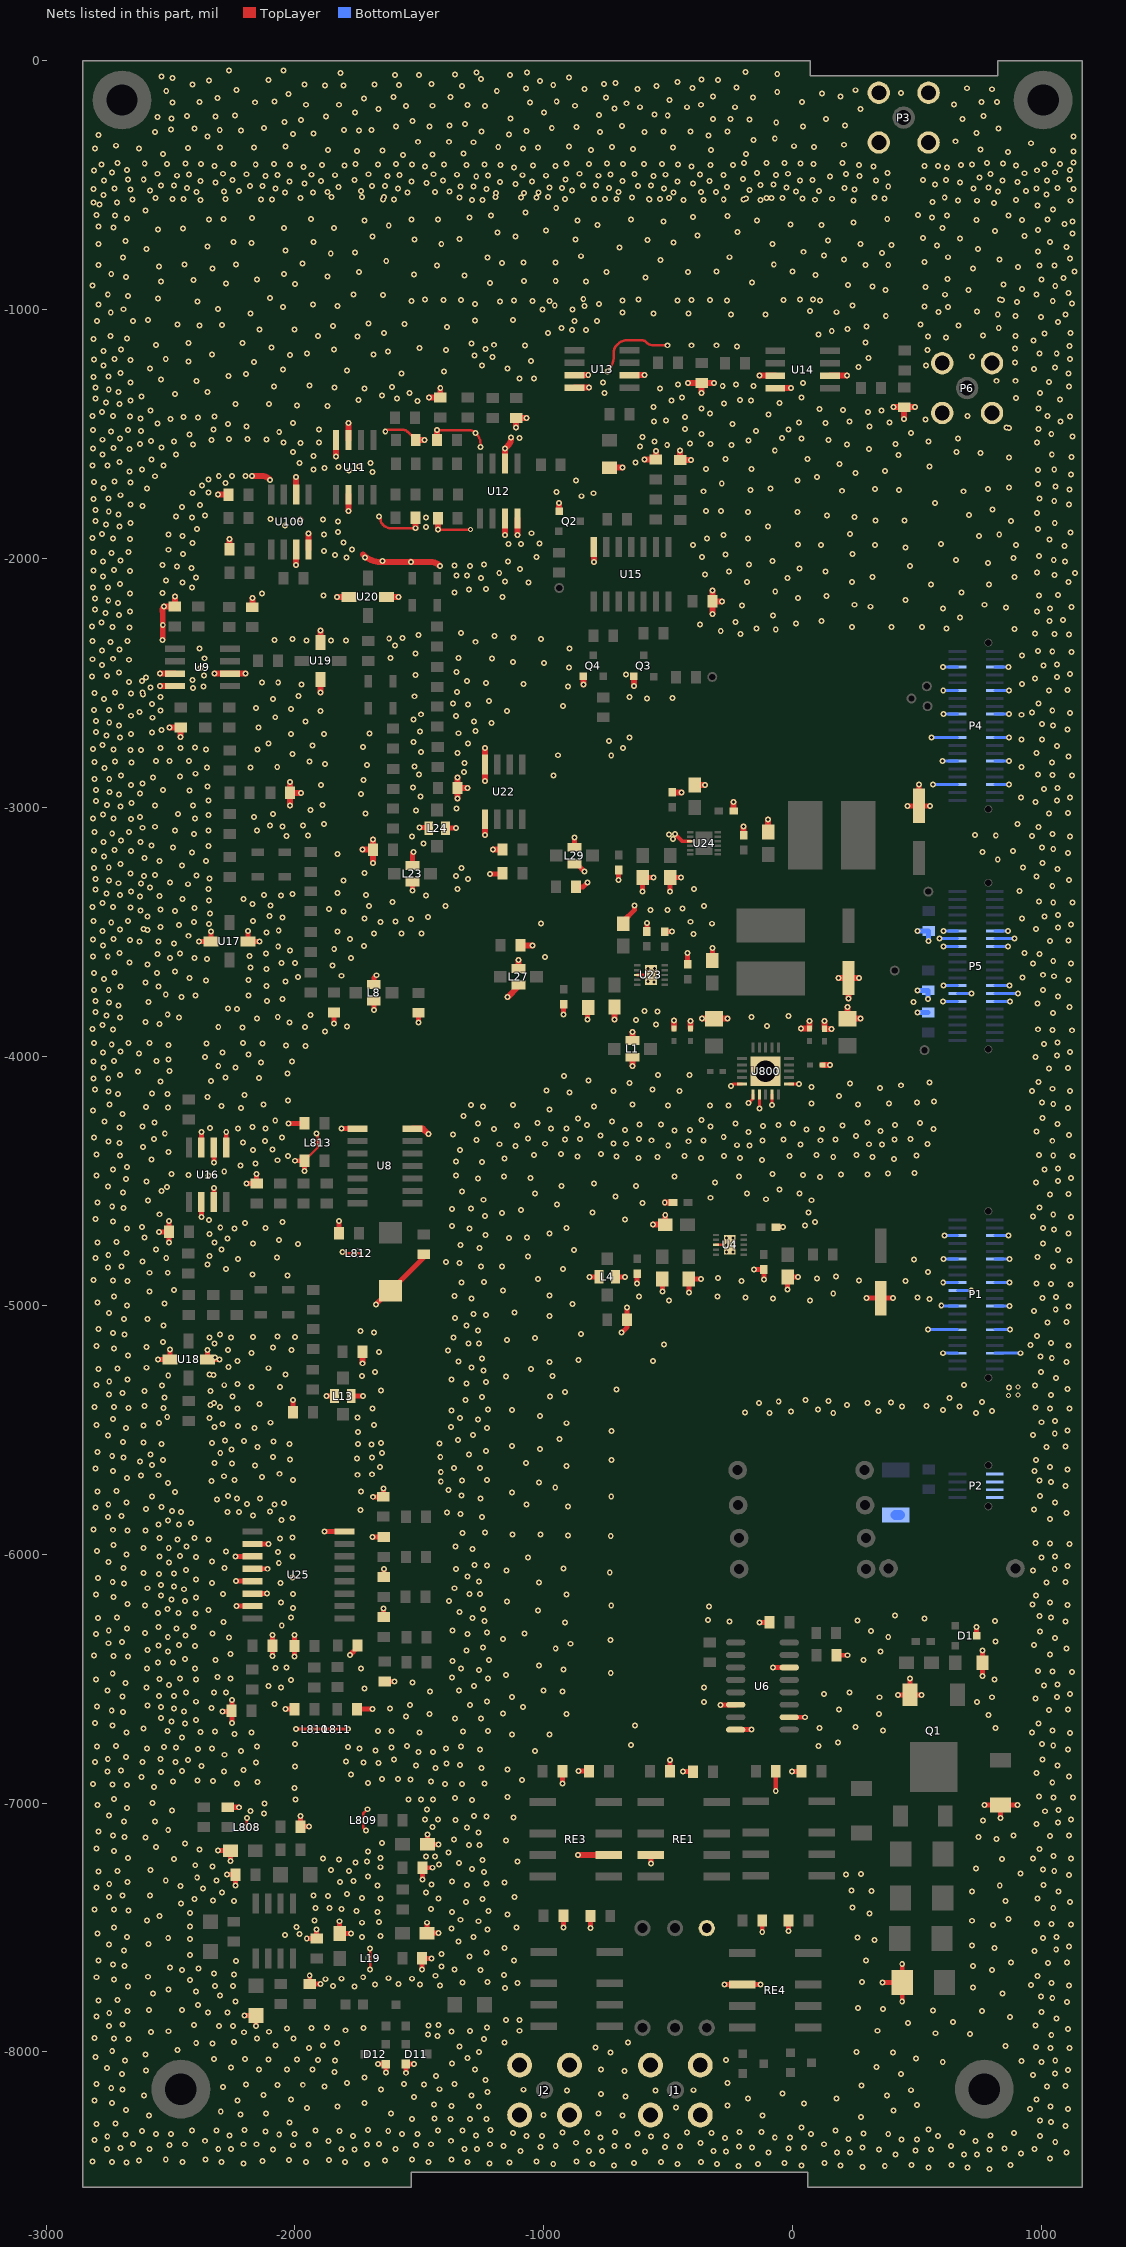
[diagram p0: the nets of this part, all layers, seen from the top]
# Altium PCB MISC109560.PcbDoc (part 3 of 7)
Units mil, origin at the board's own origin, x right, y up, seen from the top; angles counter-clockwise.
Board outline 4015.75 x 8543.31 mil, 4 copper layers (TopLayer, GND, SIG3, BottomLayer); 280 components, 173 nets, 936 pads, 3695 vias.

## Via types
v1: diameter 24, hole 12, TopLayer to BottomLayer, 3659 vias
v2: diameter 20, hole 12, TopLayer to BottomLayer, 32 vias
v3: diameter 40, hole 20, TopLayer to BottomLayer, 4 vias

## Nets (pads, with @x,y where several pads share a name; then routed paths per layer and width w, separated by ;. In a path a pad name is that pad's centre, name@x,y a point inside that pad or via, vN(x,y) a via of type N, cw(c..) or ccw(c..) an arc to the next point about the centre after c; other vN are vias at no path point) (continued)
GND: C5.1 C6.2 C7.1 C8.1 C9.2 C10.2 C11.2 C12.1 C13.2 C14.2 C15.1 C18.2 C20.1 C21.1 C31.1 C32.1 C34.1 C35.1 C36.2 C37.2 C39.2 C40.2 C42.2 C43.1 C44.2 C45.2 C46.2 C47.1 C48.1 C49.2 C50.2 C57.2 C60.2 C61.1 C62.1 C63.1 C64.1 C65.2 C66.1 C70.1 C71.1 C72.2 C73.1 C74.1 C75.1 C80.1 C81.1 C83.2 C84.2 C85.1 C86.2 C88.1 C89.2 C90.2 C93.1 C94.1 C95.2 C96.2 C97.2 C98.2 C99.1 C100.2 C101.2 C102.2 C103.1 C104.2 C105.1 C106.2 C107.2 C109.2 C110.1 C111.1 C112.2 C113.2 C114.1 C115.1 C117.1 C118.2 C119.2 C122.2 C123.2 C124.1 C125.1 C128.1 C129.1 C130.2 C800.2 C801.2 C802.2 C803.2 C804.2 C805.2 C806.2 C809.2 C888.2 D1.3 D2.2 D11.2 D12.1 J1.1 J1.2 J1.3 J1.4 J2.1 J2.2 J2.3 J2.4 L1.2 L1.4 L2.2 L4.2 L4.4 L8.2 L8.4 L13.2 L13.4 L15.2 L16.1 L19.2 L23.2 L23.4 L24.2 L24.4 L27.2 L27.4 L29.2 L29.4 L808.2 L809.2 L810.2 L811.2 L812.2 L813.2 P1.5 P1.6 P1.11 P1.12 P1.17 P1.18 P1.20 P1.23 P1.24 P1.29 P1.30 P1.35 P1.36 P2.1 P2.3 P2.5 P2.7 P3.1 P3.2 P3.3 P3.4 P4.5 P4.6 P4.11 P4.12 P4.17 P4.18 P4.23 P4.24 P4.29 P4.30 P4.35 P4.36 P5.11 P5.12 P5.13 P5.14 P5.15 P5.16 P5.25 P5.26 P5.27 P5.28 P5.29 P5.30 P6.1 P6.2 P6.3 P6.4 Q1.2 Q2.1 Q3.1 Q4.1 R13.2 R14.2 R20.2 R32.2 R53.1 R59.1 R61.1 R71.2 R72.2 R74.1 R80.2 R81.2 R82.1 R83.1 RE1.3 RE3.6 RE4.2 U4.8 U4.11 U6.6 U6.8 U6.10 U6.14 U8.7 U8.8 U9.2 U9.7 U9.8 U11.2 U11.7 U11.8 U12.2 U12.7 U12.8 U13.2 U13.7 U13.8 U14.2 U14.7 U14.8 U15.14 U16.2 U16.3 U16.5 U16.6 U16.7 U17.2 U17.4 U18.2 U18.4 U19.2 U19.4 U20.2 U20.4 U22.4 U22.5 U23.8 U23.11 U24.9 U25.2 U25.3 U25.4 U25.5 U25.6 U25.7 U25.16 U100.2 U100.7 U100.8 U800.5 U800.6 U800.7 U800.9 U800.11 U800.21 | length 17582.9
  TopLayer w10: L808.2@-2193.26,-7104.89 v1(-2193.26,-7059.26) ; C89.2@-1961.96,-4419.31 -1908.26,-4365.61 L813.2@-1908.26,-4352.89 ; v1(-1914,-4310.31) -1908.26,-4316.05 L813.2@-1908.26,-4352.89 ; L813.2@-1908.26,-4339.11 L813.2@-1908.26,-4352.89 ; v1@-1803.43,-4790.57 L812.2@-1749.85,-4790.57 L812.2@-1736.07,-4790.57 ; v1(-1714,-7110) -1725.74,-7098.26 L809.2@-1725.74,-7063.11 -1725.74,-7042.74 v1(-1708,-7025) ; v1(-1698.26,-7669.74) L19.2@-1698.26,-7617.11 v1(-1698.26,-7584.74) ; v1@-1656,-1840.17 ccw(c-1621.86,-1840.17) -1646,-1864.31 ccw(c-1613.19,-1831.5) -1613.19,-1877.9 v1(-1516.41,-1877.9) ; v1@-1638,-1488.31 cw(c-1623.51,-1502.79) -1623.51,-1482.31 -1566,-1482.31 cw(c-1566,-1507.78) -1547.99,-1489.77 C62.1@-1514.41,-1523.35 ccw(c-1539.64,-1523.35) C62.1@-1521.8,-1505.51 ; v1(-1428.41,-1483.9) -1298.13,-1483.9 cw(c-1298.13,-1519.44) -1273,-1494.31 cw(c-1318.87,-1540.18) -1254,-1540.18 v1@-1254,-1552.31 ; v1@-1423.59,-1882.31 ccw(c-1423.59,-1885.72) v1(-1426,-1883.31) v2(-1294,-1883.31) ; v1@-743,-1244.68 ccw(c-800.94,-1186.74) -719,-1186.74 -719,-1171.68 cw(c-677.96,-1171.68) -706.98,-1142.66 -702,-1137.68 cw(c-665.79,-1173.89) -665.79,-1122.68 -605.9,-1122.68 cw(c-605.9,-1146.58) -589,-1129.68 ccw(c-557.62,-1098.29) -557.62,-1142.68 v1(-503,-1142.68) ; U4.8@-308.14,-4756.94 U4.11@-252.57,-4756.94
  TopLayer w12: v1(-1994.74,-6703.26) -1811,-6703.26 ; L811.2@-1822.11,-6703.26 -1811,-6703.26 ; v1(-1786.74,-6703.26) -1811,-6703.26 ; U23.8@-625.14,-3672.94 U23.11@-590.06,-3672.94 ; -444,-3134 -442.55,-3135.45 -441.55,-3135.45 ; v1(-248,-4119) -239.67,-4110.67 U800.5@-203,-4110.67 ; v1(-177,-4188) -159.69,-4170.69 U800.6@-159.69,-4153.98 ; v1(-134.1,-4209.9) U800.7@-134.1,-4153.98 ; v1(-82.92,-4194.92) U800.9@-82.92,-4153.98 ; U800.11@-14.02,-4110.67 v1(26.33,-4110.67)
  TopLayer w13: -441.55,-3135.45 U24.9@-411.41,-3135.45
  TopLayer w16: v1(-472,-3106) -444,-3134
  TopLayer w20: v1(-2549.55,-5217.72) U18.4@-2501.92,-5217.72 v1(-2501.92,-5178.35) ; v1(-2545.96,-4705.31) R53.1@-2505.96,-4705.31 ; v1(-2505.96,-4748.31) R53.1@-2505.96,-4705.31 ; v1(-2505.96,-4662.31) R53.1@-2505.96,-4705.31 ; v1(-2385.59,-3537.72) U17.4@-2337.96,-3537.72 v1(-2337.96,-3498.27) ; v1(-2375.92,-4646.27) U16.2@-2375.92,-4585.72 ; U16.7@-2375.92,-4365.72 v1(-2375.92,-4304.35) ; v1(-2351.92,-5180.27) U18.2@-2351.92,-5217.72 v1(-2303.37,-5217.72) ; U16.3@-2325.92,-4585.72 v1(-2325.92,-4528.27) ; v1(-2325.92,-4427.27) U16.6@-2325.92,-4365.72 ; v1(-2308.89,-7191.41) C86.2@-2259.26,-7191.41 v1(-2259.26,-7233.22) ; v1(-2290.76,-6632.31) R82.1@-2253.29,-6632.31 ; U16.5@-2275.92,-4365.72 v1(-2275.92,-4303.27) ; v1(-2273.48,-7288) C83.2@-2238.48,-7288 v1(-2238.48,-7332) ; v1(-2253.29,-6679.21) R82.1@-2253.29,-6632.31 ; v1(-2253.29,-6585.77) R82.1@-2253.29,-6632.31 ; v1(-2238.61,-6008.69) U25.3@-2170.71,-6008.69 ; v1(-2236.24,-6108.69) U25.5@-2170.71,-6108.69 ; v1(-2234.24,-6208.69) U25.7@-2170.71,-6208.69 ; v1(-2201.89,-7853.41) R61.1@-2156.44,-7853.41 v1(-2156.44,-7894.96) ; v1(-2193.96,-4510.31) C47.1@-2153.96,-4510.31 v1(-2153.96,-4472.31) ; v1(-2187.96,-3495.35) U17.2@-2187.96,-3537.72 v1(-2141.41,-3537.72) ; U25.6@-2170.71,-6158.69 v1(-2111.24,-6158.69) ; U25.4@-2170.71,-6058.69 v1(-2109.24,-6058.69) ; U25.2@-2170.71,-5958.69 v1(-2106.24,-5958.69) ; v1(-2090.71,-6409.79) -2090.71,-6396.01 ; R83.1@-2090.71,-6367.69 -2090.71,-6396.01 ; v1(-2090.71,-6324.23) -2090.71,-6396.01 ; v1(-2037.93,-6623.01) C105.1@-2000.93,-6623.01 ; v1(-2025,-4270) -1995.65,-4270 -1994.96,-4269.31 C50.2@-1960.96,-4269.31 ; C64.1@-2007,-5429.96 v1(-2007,-5380.96) ; v1(-2001.93,-6412.01) C128.1@-2001.93,-6369.01 v1(-2001.93,-6324.01) ; v1(-1999.96,-4419.31) C89.2@-1961.96,-4419.31 v1(-1961.96,-4461.31) ; v1(-1978.48,-7052) R74.1@-1978.48,-7095 v1(-1943.48,-7095) ; v1(-1952.48,-7544) C75.1@-1912.48,-7544 v1(-1912.48,-7508) ; v1(-1940.44,-7692.96) R59.1@-1940.44,-7727.41 v1(-1896.89,-7727.41) ; v1(-1881,-5908.69) U25.16@-1800.71,-5908.69 ; v1(-1873.83,-5364.83) L13.2@-1840.46,-5364.83 ; v1(-1842.59,-3868.72) C48.1@-1842.59,-3826.27 ; C104.2@-1822.96,-4711.31 v1(-1822.96,-4661.04) ; v1(-1820.48,-7475) C71.1@-1820.48,-7524 v1(-1775.48,-7524) ; v1(-1812,-4290.35) U8.8@-1748.37,-4290.35 ; v1(-1778.93,-6405.01) C129.1@-1747.93,-6374.01 ; L13.4@-1773.54,-5364.83 v1(-1725.83,-5364.83) ; C90.2@-1749.93,-6623.01 v1(-1688.93,-6623.01) ; v1(-1687.52,-5931.42) C102.2@-1643.89,-5931.42 ; v1(-1685.34,-5769.42) C96.2@-1644.89,-5769.42 v1(-1644.89,-5736.05) ; v1(-1682.83,-3812.83) L8.4@-1682.83,-3777.46 ; L8.2@-1682.83,-3710.54 -1682.83,-3684.83 v1(-1672,-3674) ; v1(-1675,-4997) -1619.16,-4941.16 C49.2@-1616,-4941.16 -1483,-4808.16 C888.2@-1483,-4795 ; v1(-1665.48,-8049) D12.1@-1634.48,-8049 v1(-1634.48,-8083) ; C118.2@-1643.93,-6252.01 v1(-1643.93,-6218.01) ; C109.2@-1642.89,-6092.42 v1(-1642.89,-6060.05) ; C130.2@-1639.93,-6511.01 v1(-1599.93,-6511.01) ; v1(-1554.26,-8083.78) D11.2@-1554.26,-8048.69 v1(-1521.79,-8048.69) ; v1(-1527.83,-3333.83) L23.4@-1527.83,-3299.46 ; L23.2@-1527.83,-3232.54 v1@-1527.83,-3182.14 ; v1(-1503.43,-3864.61) C123.2@-1503.43,-3824.61 ; v1(-1500,-3081) L24.4@-1464.24,-3081 ; v1(-1488.48,-7668) C74.1@-1488.48,-7624 v1(-1450.48,-7624) ; v1(-1487.48,-7307) C72.2@-1487.48,-7260 v1(-1447.48,-7260) ; v1(-1468.48,-7481) C70.1@-1468.48,-7523 v1(-1422.48,-7523) ; v1(-1467.48,-7126) C73.1@-1467.48,-7166 v1(-1423.48,-7166) ; L24.2@-1395.54,-3082.78 v1@-1353.78,-3082.78 ; v1(-1216,-3268) C125.1@-1169.31,-3268 ; v1(-925,-6920.59) C32.1@-925,-6872.59 ; v1(-921,-7500.59) C39.2@-921,-7453.59 ; v1(-920,-3832) C98.2@-920,-3790 ; L29.4@-876.83,-3226.46 -867.54,-3226.46 v1(-837,-3257) ; L29.2@-876.83,-3159.54 v1(-876.83,-3119.83) ; C115.1@-871,-3319 -842,-3319 v1(-825,-3302) ; v1(-861.41,-6872) C31.1@-817.66,-6872 ; v1(-824,-3851) -824,-3805.31 C93.1@-822,-3803.31 ; v1(-816.17,-4885.83) L4.2@-778.46,-4885.83 ; v1(-812.96,-7501.55) C40.2@-812.96,-7454 ; L4.4@-711.54,-4885.83 v1(-672.83,-4885.83) ; v1(-699,-3291) C113.2@-699,-3251 ; v1(-687,-5110) -665,-5088 C13.2@-665,-5059 v1(-665,-5009) ; C101.2@-680,-3467 -680,-3456 -635,-3411 v1(-635,-3393) ; v1(-625,-4912) C11.2@-625,-4873 ; v1(-603,-3337) C114.1@-603,-3282 v1(-559,-3282) ; R72.2@-586,-3498 v1(-586,-3464) ; v1(-569.66,-7242.25) RE1.3@-569.66,-7208.6 ; v1(-524,-4944) C12.1@-524,-4895 ; R71.2@-514,-3499 v1(-484,-3499) ; C21.1@-493,-6871.59 v1(-493,-6826.59) ; v1(-492,-3337) C110.1@-492,-3282 v1(-449,-3282) ; v1(-440,-6873.59) C20.1@-401,-6873.59 ; C95.2@-422,-3630 v1(-422,-3584) ; v1(-417,-4948) C7.1@-417,-4895 v1(-369,-4895) ; C94.1@-323,-3615 v1(-323,-3565) ; v1(-289.69,-6605.31) U6.6@-229,-6605.31 ; v1(-273.98,-7728.57) RE4.2@-202,-7728.57 v1(-129.02,-7728.57) ; U6.8@-229,-6705.31 v1(-165.31,-6705.31) ; v1(-156,-4856) C9.2@-116,-4856 v1(-116,-4897) ; v1(-134,-6273.69) C15.1@-93,-6273.69 ; v1(-122.26,-7517.33) C35.1@-122.26,-7472 ; v1(-79.69,-6455.31) U6.14@-13.6,-6455.31 ; v1(-68,-6952.59) C37.2@-68,-6872.59 ; R13.2@-67,-4686 v1(-39,-4686) ; v1(-20,-4936) C8.1@-20,-4887 v1(22,-4887) ; v1(-17.26,-7514.33) C34.1@-17.26,-7472 ; U6.10@-13.6,-6655.31 v1(48.69,-6655.31) ; v1(-2,-6872.59) C36.2@35,-6872.59 ; C18.2@175.81,-6406.2 v1(220.51,-6406.2) ; v1(296.76,-4971.24) C10.2@354,-4971.24 v1(403.24,-4971.24) ; v1(360.31,-7720.99) D2.2@440.22,-7720.99 ; v1(423,-6565) Q1.2@472,-6565 ; v1(440.22,-7796.53) D2.2@440.22,-7720.99 ; v1(440.22,-7647.53) D2.2@440.22,-7720.99 ; v1(462,-2993) C117.1@508,-2993 ; v1(472,-6499) Q1.2@472,-6565 ; v1(508,-2908) C117.1@508,-2993 ; v1(517,-6565) Q1.2@472,-6565 ; v1(552,-2993) C117.1@508,-2993 ; D1.3@739,-6328 v1(739,-6293) ; L2.2@762.78,-6436.31 v1(762.78,-6386.22) ; v1(763,-6488.91) L2.2@763,-6444 ; v1(771,-7008) C6.2@835,-7008 ; v1(835,-7061) C6.2@835,-7008 ; v1(903,-7008) C6.2@835,-7008
  TopLayer w24: v1(-2543.04,-2462.27) U9.7@-2481.59,-2462.27 ; v1(-2541.96,-2512.27) U9.8@-2481.59,-2512.27 ; v1@-2531,-2323.31 -2531,-2214.09 ccw(c-2537.83,-2214.09) -2533,-2209.26 ; v1(-2503.59,-2677.72) C66.1@-2458.96,-2677.72 v1(-2458.96,-2717.27) ; v1(-2482.59,-2151.72) C42.2@-2482.59,-2192.27 v1(-2525.96,-2192.27) ; v1(-2322.96,-2462.27) U9.2@-2261.59,-2462.27 v1(-2197.96,-2462.27) ; v1(-2309.59,-1742.72) C43.1@-2265.96,-1742.72 ; C809.2@-2269,-7017 v1(-2224,-7017) ; C61.1@-2263,-1962.31 v1(-2263,-1921.31) ; v1(-2172,-1667.31) -2133.38,-1667.31 cw(c-2133.38,-1711.69) v1@-2102,-1680.31 ; C60.2@-2170.59,-2195.27 v1(-2170.59,-2158.72) ; v1(-2019,-2992.31) C65.2@-2019,-2941.31 ; v1(-2019,-2898.31) C65.2@-2019,-2941.31 ; v1(-1994.96,-2025.27) U100.7@-1994.96,-1962.72 ; U100.2@-1994.96,-1742.72 v1(-1994.96,-1672.35) ; v1(-1975,-2941.31) C65.2@-2019,-2941.31 ; U100.8@-1944.96,-1962.72 v1(-1944.96,-1899.35) ; v1(-1897,-2538.31) U19.2@-1897,-2486.31 ; U19.4@-1897,-2336.31 v1(-1897,-2289.31) ; v1(-1834.41,-1588.9) U11.8@-1834.41,-1523.35 ; v1(-1830,-2153.31) U20.4@-1782,-2153.31 ; v1(-1784.41,-1807.72) U11.2@-1784.41,-1743.35 ; U11.7@-1784.41,-1523.35 v1(-1784.41,-1455.9) ; v1(-1728.73,-5233) C122.2@-1728.73,-5186 ; v1(-1728,-3169.31) C84.2@-1686,-3169.31 ; -1726.29,-1984.02 ccw(c-1655.58,-1913.31) -1655.58,-2013.31 -1552,-2013.31 ; v1(-1686,-3222.31) C84.2@-1686,-3169.31 ; v1(-1686,-3129.31) C84.2@-1686,-3169.31 ; U20.2@-1632,-2153.31 v1(-1584,-2153.31) ; v1@-1536.41,-2012.31 cw(c-1536.41,-2015.72) v1(-1534,-2013.31) -1552,-2013.31 ; U8.7@-1528.37,-4290.35 -1485.65,-4290.35 v1(-1464,-4312) ; v1(-1516.41,-1877.9) C44.2@-1516.41,-1835.35 ; C62.1@-1514.41,-1523.35 v1(-1479.04,-1523.35) ; v1(-1461,-1353.31) C80.1@-1416,-1353.31 v1(-1416,-1314.31) ; C63.1@-1428.41,-1523.35 v1(-1428.41,-1483.9) ; v1(-1426,-1883.31) C45.2@-1426,-1838.31 ; v1@-1420,-2027.31 ccw(c-1453.8,-2061.11) -1453.8,-2013.31 -1552,-2013.31 ; v1(-1346,-2963.61) C85.1@-1346,-2921.61 ; v1(-1346,-2878.61) C85.1@-1346,-2921.61 ; v1(-1307,-2921.61) C85.1@-1346,-2921.61 ; v1(-1236.69,-3110) U22.5@-1236.69,-3047 ; v1(-1236.69,-2894) U22.4@-1236.69,-2827 v1(-1236.69,-2761) ; v1(-1204.69,-3168.69) C124.1@-1166,-3168.69 ; v1(-1156,-1905.31) U12.7@-1156,-1838.31 ; U12.2@-1156,-1618.31 v1(-1156,-1558.31) -1143.73,-1546.03 ccw(c-1174.46,-1515.31) v1@-1131,-1515.31 ; v1(-1145,-3762) -1101.83,-3718.83 L27.4@-1101.83,-3713.46 ; v1(-1111,-1472.31) C81.1@-1111,-1434.31 v1(-1069,-1434.31) ; v1(-1106,-1904.31) U12.8@-1106,-1838.31 ; L27.2@-1101.83,-3646.54 v1(-1101.83,-3612.17) ; C100.2@-1093,-3555 v1(-1046,-3555) ; Q2.1@-938.59,-1809.27 v1(-938.59,-1776.9) ; U13.8@-875.96,-1313.09 v1(-818.41,-1313.09) ; U13.7@-875.96,-1263.09 v1(-821.41,-1263.09) ; v1(-862.01,-7208.6) RE3.6@-739.31,-7208.6 ; v1(-841,-2505.31) Q4.1@-841,-2472.31 ; v1(-798.96,-2014.27) U15.14@-798.96,-1952.72 ; L15.2@-736,-1634 v1(-683,-1634) ; v1(-716,-3851) C99.1@-716,-3802.31 ; U13.2@-655.96,-1263.09 v1(-595.59,-1263.09) ; v1(-643.83,-4039.17) L1.4@-643.83,-4003.46 ; L1.2@-643.83,-3936.54 v1(-643.83,-3902.17) ; v1(-638,-2512.31) Q3.1@-638,-2473.31 ; v1(-596,-1602.31) C57.2@-550,-1602.31 v1(-550,-1568.31) ; v1(-562,-4676) C14.2@-512,-4676 v1(-512,-4637) ; v1(-514,-4587) R14.2@-481,-4587 ; R81.2@-484,-2939 v1(-446,-2939) ; C806.2@-477,-3888.31 v1(-477,-3856) ; v1(-452,-1565.31) C46.2@-452,-1604.31 v1(-409,-1604.31) ; v1(-421,-1294.68) L16.1@-366,-1294.68 ; C805.2@-410,-3888.31 v1(-410,-3857) ; C119.2@-393,-2910 v1(-352,-2910) ; v1(-366,-1334.68) L16.1@-366,-1294.68 ; v1(-363.69,-3848.31) C804.2@-316,-3848.31 v1(-262.31,-3848.31) ; v1(-323,-2223.31) C88.1@-323,-2171.31 ; v1(-323,-2127.31) C88.1@-323,-2171.31 ; v1(-316,-1294.68) L16.1@-366,-1294.68 ; v1(-284,-2171.31) C88.1@-323,-2171.31 ; R80.2@-237,-3014 v1(-237,-2977) ; C112.2@-197,-3111 v1(-197,-3076) ; v1(-133.59,-1265.09) U14.7@-69.96,-1265.09 ; C111.1@-99,-3099 v1(-99,-3049) ; U14.8@-69.96,-1315.09 v1(-7.59,-1315.09) ; v1(32.69,-3888.31) C801.2@67,-3888.31 v1(67,-3857) ; C803.2@120,-4034 v1(150,-4034) ; v1(127,-3857) C802.2@127,-3889.31 v1(155.69,-3889.31) ; U14.2@150.04,-1265.09 v1(217.59,-1265.09) ; v1(184.24,-3685.24) C97.2@224,-3685.24 ; v1(220,-3801) C800.2@220,-3848 v1(272,-3848) ; v1(224,-3767) C97.2@224,-3685.24 ; v1(265.76,-3685.24) C97.2@224,-3685.24 ; v1(405,-1391.68) R32.2@448,-1391.68 ; v1(448,-1438.68) R32.2@448,-1391.68 ; v1(492,-1391.68) R32.2@448,-1391.68 ; -2533,-2209.26 cw(c-2508.97,-2209.26) v1(-2525.96,-2192.27) ; -2533,-2209.26 cw(c-2508.97,-2209.26) v1(-2525.96,-2192.27)
  BottomLayer w12: v1(543.06,-5098.25) P1.30@662.43,-5098.25 ; v1(558.02,-2719.28) P4.24@662.43,-2719.28 ; v1(564.05,-2908.26) P4.36@662.43,-2908.26 ; v1(590.39,-3526.91) P5.14@662.43,-3526.91 ; v1(597,-5000.31) 600.46,-5003.76 P1.24@662.43,-5003.76 ; v1(602.54,-2813.77) P4.30@662.43,-2813.77 ; v1(603.43,-3778.88) P5.30@662.43,-3778.88 ; v1(603.51,-2435.82) P4.6@662.43,-2435.82 ; v1(604.57,-5192.74) P1.36@662.43,-5192.74 ; v1(604.97,-4909.28) P1.18@662.43,-4909.28 ; v1(605,-2530.31) P4.12@662.43,-2530.31 ; v1(605.1,-3558.41) P5.16@662.43,-3558.41 ; v1(605.11,-3495.42) P5.12@662.43,-3495.42 ; v1(605.49,-2624.8) P4.18@662.43,-2624.8 ; v1(606.42,-3715.89) P5.26@662.43,-3715.89 ; v1(606.48,-4814.79) P1.12@662.43,-4814.79 ; v1(609.99,-4720.3) P1.6@662.43,-4720.3 ; P1.20@662.43,-4940.77 v1(717.54,-4940.77) ; P5.28@662.43,-3747.39 v1(717.92,-3747.39) ; P1.35@812.04,-5192.74 v1(915.43,-5192.74) ; P1.29@812.04,-5098.25 v1(872.94,-5098.25) ; P1.23@812.04,-5003.76 v1(871.46,-5003.76) ; P1.17@812.04,-4909.28 v1(871.97,-4909.28) ; P1.11@812.04,-4814.79 v1(871.52,-4814.79) ; P1.5@812.04,-4720.3 v1(867.99,-4720.3) ; P5.29@812.04,-3778.88 v1(872.57,-3778.88) ; P5.27@812.04,-3747.39 v1(905.92,-3747.39) ; P5.25@812.04,-3715.89 v1(870.42,-3715.89) ; P5.15@812.04,-3558.41 v1(865.1,-3558.41) ; P5.13@812.04,-3526.91 v1(891.39,-3526.91) ; P5.11@812.04,-3495.42 v1(864.89,-3495.42) ; P4.35@812.04,-2908.26 v1(868.95,-2908.26) ; P4.29@812.04,-2813.77 v1(869.46,-2813.77) ; P4.23@812.04,-2719.28 v1(868.98,-2719.28) ; P4.17@812.04,-2624.8 v1(869.49,-2624.8) ; P4.11@812.04,-2530.31 v1(870,-2530.31) ; P4.5@812.04,-2435.82 v1(866.51,-2435.82)
  BottomLayer w20: v1(501,-3824.31) C106.2@544,-3824.31 ; v1(501,-3734.31) C103.1@544,-3734.31 v1(544,-3769.31) ; v1(501,-3496.31) C107.2@546,-3496.31 v1(546,-3536.31)
  BottomLayer w40: C5.1@414,-5842.31 C5.1@432,-5842.31